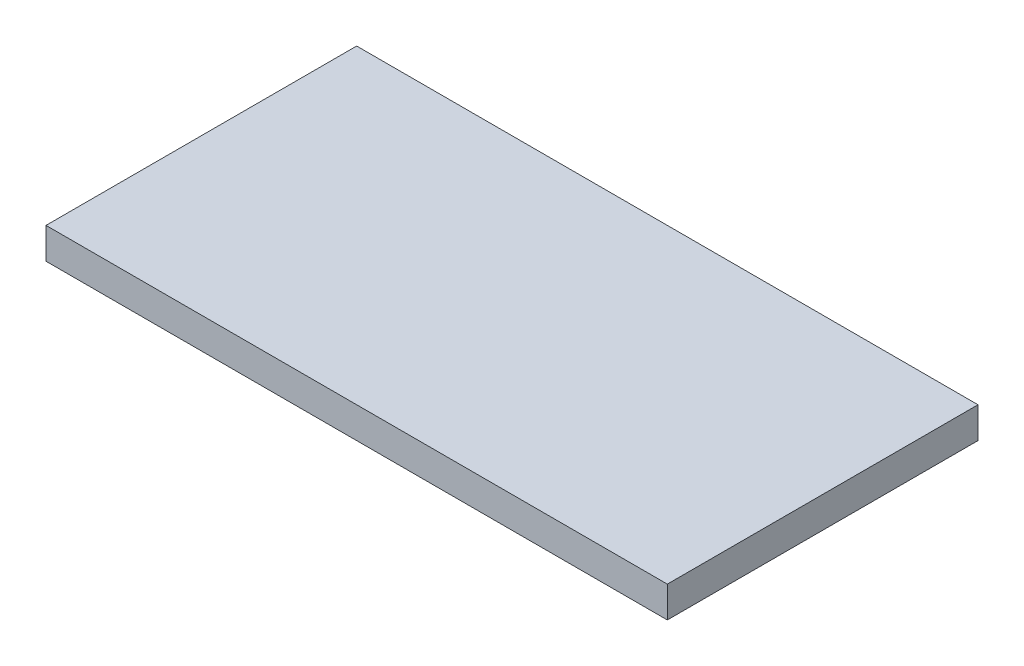
from build123d import *

# Parameters (mm, degrees)
SKETCH_1_W      = 1000
SKETCH_1_H      = 500
EXTRUDE_1_DEPTH = 50


with BuildPart() as part:
    # 草图1 → 凸台-拉伸1 (new body)
    with BuildSketch(Plane(origin=(0, 0, 0), x_dir=(1, 0, 0), z_dir=(0, 1, 0))):
        Rectangle(SKETCH_1_W, SKETCH_1_H)
    extrude(amount=EXTRUDE_1_DEPTH)


solid = part.part
